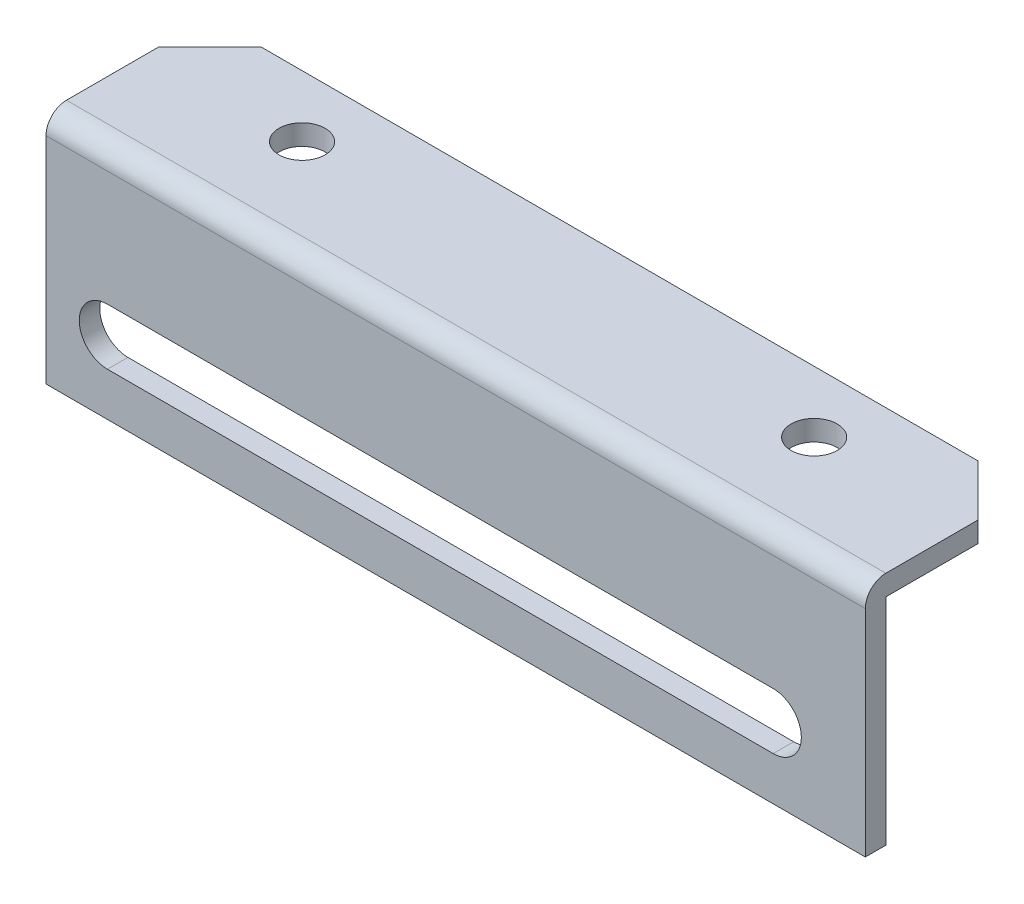
SolidWorks part; units mm, degrees
ref_plane "Front Plane" through (0, 0, 0) normal (0, 0, 1) x (1, 0, 0)
ref_plane "Top Plane" through (0, 0, 0) normal (0, 1, 0) x (1, 0, 0)
ref_plane "Right Plane" through (0, 0, 0) normal (1, 0, 0) x (0, 0, -1)
ref_plane "Plane 4" through (0, 0, 0) normal (0, 0, -1) x (-1, 0, 0)
sketch "Sketch 1" plane through (0, 0, 0) normal (0, 0, -1) x (-1, 0, 0)
  line L0 (75, 12.5) -> (-75, 12.5)
  line L1 (-75, 12.5) -> (-75, -12.5)
  line L2 (-75, -12.5) -> (75, -12.5)
  line L3 (75, -12.5) -> (75, 12.5)
extrude "Boss-Extrude 1" add sketch "Sketch 1" against normal blind 18
sketch "Sketch 2" plane through (-75, 0, 0) normal (-1, 0, 0) x (0, 0, 1)
  line L0 (16, -12.5) -> (16, 10.5)
  line L1 (16, 10.5) -> (0, 10.5)
  line L2 (0, 10.5) -> (0, -12.5)
  line L3 (0, -12.5) -> (16, -12.5)
extrude "Cut-Extrude 1" cut sketch "Sketch 2" against normal through all
sketch "Sketch 4" plane through (0, 0, 18) normal (0, 0, 1) x (1, 0, 0)
  line L0 (-69, -6.25) -> (-4, -6.25)
  line L1 (-4, -0.75) -> (-69, -0.75)
  line L2 (-75, 12.5) -> (75, 12.5) construction
  arc A0 (-4, -6.25) -> (-4, -0.75) centre (-4, -3.5) ccw
  arc A1 (-69, -0.75) -> (-69, -6.25) centre (-69, -3.5) ccw
  dimension "D1" = 16
extrude "Cut-Extrude 3" cut sketch "Sketch 4" against normal through all
hole_wizard "Ø4.5 (4.5) Hole 1" positions "Sketch 6" profile "Sketch 5" hole size "Ø4.5" standard "GB"
sketch "Sketch 6" plane through (0, 12.5, 0) normal (0, 1, 0) x (-1, 0, 0)
  line L0 (75, 18) -> (-75, 18) construction
  point P0 (-60, 8)
  dimension "D1" = 10
sketch "Sketch 5" plane through (60, 12.5, 8) normal (1, 0, 0) x (0, 0, 1)
  line L0 (0, 0) -> (0, 16.3519)
  line L1 (0, 16.3519) -> (2.25, 15)
  line L2 (2.25, 15) -> (2.25, 0)
  line L5 (2.25, 0) -> (0, 0)
  line L10 (0, 16.3519) -> (-2.25, 15) construction
  line L11 (0, -6.35) -> (0, 107.95) construction
  dimension "鑽孔直徑" = 4.5
  dimension "鑽孔深度" = 15
  dimension "導頭角度" = 118
hole_wizard "Ø4.5 (4.5) Hole 3" positions "Sketch 8" profile "Sketch 7" hole size "Ø4.5" standard "GB"
sketch "Sketch 8" plane through (0, 12.5, 0) normal (0, 1, 0) x (-1, 0, 0)
  line L0 (75, 18) -> (-75, 18) construction
  point P0 (60, 8)
  dimension "D1" = 10
sketch "Sketch 7" plane through (-60, 12.5, 8) normal (1, 0, 0) x (0, 0, 1)
  line L0 (0, 0) -> (0, 16.3519)
  line L1 (0, 16.3519) -> (2.25, 15)
  line L2 (2.25, 15) -> (2.25, 0)
  line L5 (2.25, 0) -> (0, 0)
  line L10 (0, 16.3519) -> (-2.25, 15) construction
  line L11 (0, -6.35) -> (0, 107.95) construction
  dimension "鑽孔直徑" = 4.5
  dimension "鑽孔深度" = 15
  dimension "導頭角度" = 118
hole_wizard "Ø4.5 (4.5) Hole 2" positions "Sketch 10" profile "Sketch 9" hole size "Ø4.5" standard "GB"
sketch "Sketch 10" plane through (0, 12.5, 0) normal (0, 1, 0) x (-1, 0, 0)
  line L0 (75, 18) -> (-75, 18) construction
  circle A0 centre (60, 8) radius 2.25 construction
  point P0 (10, 8)
  dimension "D2" = 50
  dimension "D1" = 10
sketch "Sketch 9" plane through (-10, 12.5, 8) normal (1, 0, 0) x (0, 0, 1)
  line L0 (0, 0) -> (0, 16.3519)
  line L1 (0, 16.3519) -> (2.25, 15)
  line L2 (2.25, 15) -> (2.25, 0)
  line L5 (2.25, 0) -> (0, 0)
  line L10 (0, 16.3519) -> (-2.25, 15) construction
  line L11 (0, -6.35) -> (0, 107.95) construction
  dimension "鑽孔直徑" = 4.5
  dimension "鑽孔深度" = 15
  dimension "導頭角度" = 118
chamfer "Chamfer 1" distance 2 angle 45 1 edges at (75, -12.5, 17)
fillet "Fillet 1" radius 2 1 edges at (0, 12.5, 18)
sketch "Sketch 11" plane through (0, 12.5, 0) normal (0, 1, 0) x (1, 0, 0)
  line L0 (-75, -16) -> (-75, 0) construction
  line L1 (75, 0) -> (-75, 0)
  line L2 (75, 0) -> (75, -2)
  line L3 (75, -2) -> (-75, -2)
  line L4 (-75, 0) -> (-75, -2)
  dimension "D1" = 2
extrude "Cut-Extrude 4" cut sketch "Sketch 11" against normal blind 10
chamfer "Chamfer 4" distance 5 angle 45 2 edges at (75, 11.5, 2) (-75, 11.5, 2)
sketch "Sketch 12" plane through (0, 0, 2) normal (0, 0, -1) x (-1, 0, 0)
  line L0 (75, 12.5) -> (75, 10.5) construction
  line L1 (-5, -22.9293) -> (-126.932, -22.9293)
  line L2 (-5, -22.9293) -> (-5, 25.439)
  line L3 (-5, 25.439) -> (-126.932, 25.439)
  line L4 (-126.932, -22.9293) -> (-126.932, 25.439)
  dimension "D1" = 80
extrude "Cut-Extrude 5" cut sketch "Sketch 12" against normal through all
chamfer "Chamfer 5" distance 5 angle 45 1 edges at (5, 11.5, 2)
sketch "Sketch 13" plane through (0, 0, 16) normal (0, 0, -1) x (-1, 0, 0)
  line L0 (-5, 10.5) -> (-5, -12.5) construction
  line L1 (75, -12.5) -> (-5, -12.5)
  line L2 (75, -12.5) -> (75, -10.5)
  line L3 (75, -10.5) -> (-5, -10.5)
  line L4 (-5, -12.5) -> (-5, -10.5)
  dimension "D1" = 2
extrude "Cut-Extrude 6" cut sketch "Sketch 13" against normal blind 10
